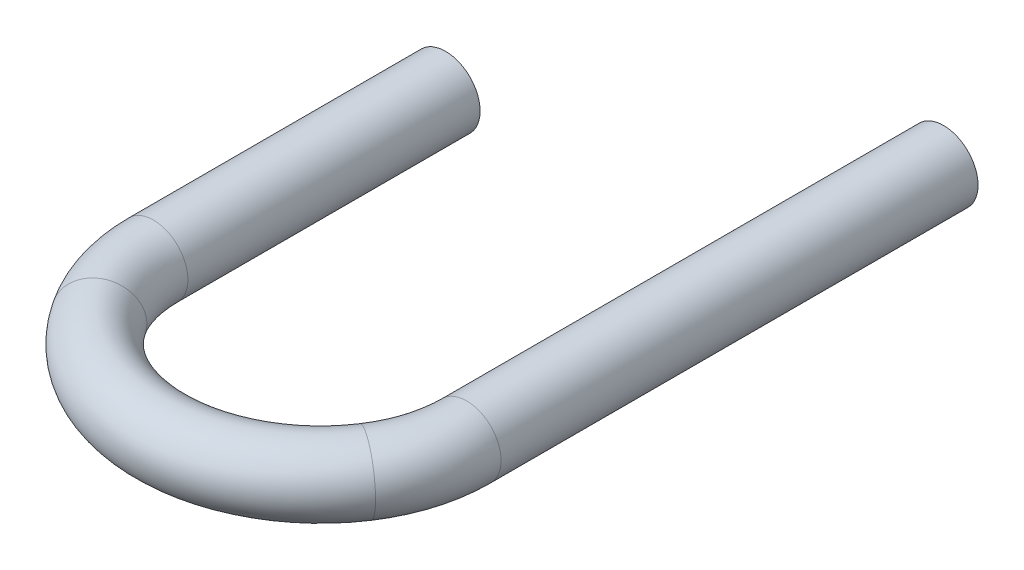
SolidWorks part; units mm, degrees
material "PE 高密度"
ref_plane "Front Plane" through (0, 0, 0) normal (0, 0, 1) x (1, 0, 0)
ref_plane "Top Plane" through (0, 0, 0) normal (0, 1, 0) x (1, 0, 0)
ref_plane "Right Plane" through (0, 0, 0) normal (1, 0, 0) x (0, 0, -1)
sketch "Sketch1" plane through (0, 0, 0) normal (0, 0, 1) x (1, 0, 0)
  circle A0 centre (0, 0) radius 11
  circle A1 centre (0, 0) radius 7.5
  dimension "D1" = 15
  dimension "D2" = 22
sketch "Sketch2" plane through (0, 0, 0) normal (0, 1, 0) x (1, 0, 0)
  line L0 (0, 0) -> (0, -93.2989)
  line L1 (100, -93.2989) -> (100, 59)
  line L3 (0, -100) -> (100, -100) construction
  arc A0 (92.5614, -118.0808) -> (7.4386, -118.0808) centre (50, -90) cw
  arc A1 (92.5614, -118.0808) -> (100, -93.2989) centre (55, -93.2989) ccw
  arc A2 (7.4386, -118.0808) -> (0, -93.2989) centre (45, -93.2989) cw
  dimension "D3" = 10
  dimension "D4" = 45
  dimension "D1" = 100
  dimension "D2" = 100
  dimension "D5" = 152.2989
sweep "Sweep1" add profiles "Sketch1" path "Sketch2"
